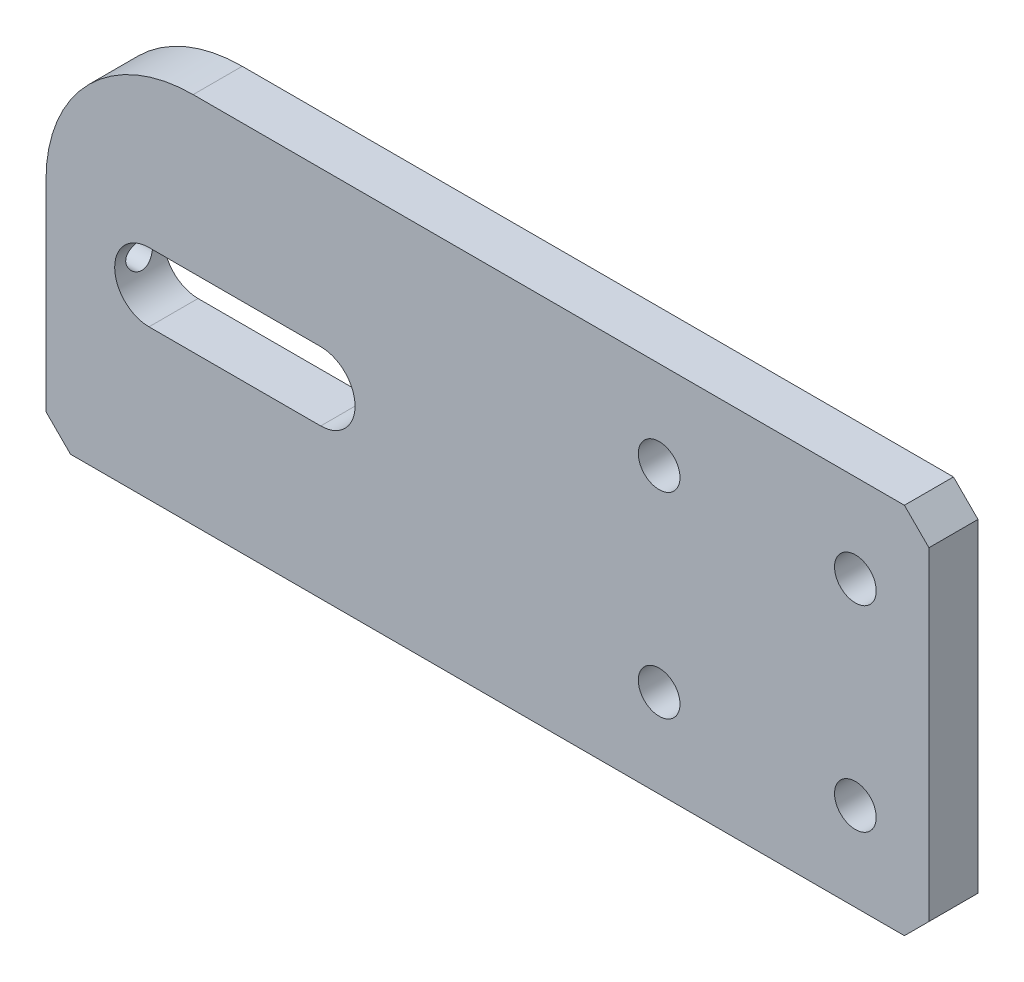
from build123d import *

# Parameters (mm, degrees)
EXTRUDE_1_DEPTH              = 5
HOLE_WIZARD_8_5_8_5_1_D      = 8.5
PATTERN_LINEAR_1_COUNT       = 2
PATTERN_LINEAR_1_PITCH       = 40
MIRROR_1_COPY_1_D            = 8.5
CUT_EXTRUDE_1_DEPTH          = 10
HOLE_WIZARD_5_5_5_5_1_REACH  = 186.035
HOLE_WIZARD_5_5_5_5_1_BORE_R = 2.75
CHAMFER_1_SIZE               = 5


with BuildPart() as part:
    # 草图2 → 凸台-拉伸1 (new, symmetric)
    with BuildSketch(Plane.XY):
        with BuildLine():
            Line((-60, 38), (90, 38))
            Line((90, 38), (90, -38))
            Line((90, -38), (-90, -38))
            Line((-90, -38), (-90, 8))
            ThreePointArc((-90, 8), (-81.213203436, 29.213203436), (-60, 38))
        make_face()
    extrude(amount=EXTRUDE_1_DEPTH, both=True)

    # Ø8.5 (8.5) 直径孔1 (through all)
    with Locations(Plane.XY.offset(5)):
        with Locations((75, 20)):
            hole_wizard_8_5_8_5_1 = Hole(HOLE_WIZARD_8_5_8_5_1_D / 2)

    # 阵列(线性)1: Ø8.5 (8.5) 直径孔1 ×2
    with Locations(*[(-i * PATTERN_LINEAR_1_PITCH, 0, 0) for i in range(1, PATTERN_LINEAR_1_COUNT)]):
        add(hole_wizard_8_5_8_5_1, mode=Mode.SUBTRACT)

    # 镜向1: Ø8.5 (8.5) 直径孔1 across plane
    add(hole_wizard_8_5_8_5_1.mirror(Plane.ZX), mode=Mode.SUBTRACT)

    # 镜向1 copy 1 (through all)
    with Locations(Plane(origin=(-40, 0, 5), x_dir=(1, 0, 0), z_dir=(0, 0, 1))):
        with Locations((75, -20)):
            Hole(MIRROR_1_COPY_1_D / 2)

    # 草图5 → 切除-拉伸1 (cut)
    with BuildSketch(Plane.XY.offset(5)):
        with BuildLine():
            Line((-69, 6.5), (-34, 6.5))
            ThreePointArc((-34, 6.5), (-27, -0.5), (-34, -7.5))
            Line((-34, -7.5), (-69, -7.5))
            ThreePointArc((-69, -7.5), (-76, -0.5), (-69, 6.5))
        make_face()
    extrude(amount=-CUT_EXTRUDE_1_DEPTH, mode=Mode.SUBTRACT)

    # Ø5.5 (5.5) 直径孔1 bore → Ø5.5 (5.5) 直径孔1 (cut, up to next)
    with BuildSketch(Plane.ZY.offset(90), mode=Mode.PRIVATE) as hole_wizard_5_5_5_5_1_sk1:
        with Locations((0, -0.5)):
            Circle(HOLE_WIZARD_5_5_5_5_1_BORE_R)
    hole_wizard_5_5_5_5_1_tool1 = extrude(hole_wizard_5_5_5_5_1_sk1.sketch, amount=-HOLE_WIZARD_5_5_5_5_1_REACH, mode=Mode.PRIVATE) & part.part
    add(hole_wizard_5_5_5_5_1_tool1.solids().sort_by_distance((-90, -0.5, 0))[0], mode=Mode.SUBTRACT)

    # 倒角1
    chamfer_1_edges = [part.edges().sort_by_distance(p)[0] for p in [
        (90, -38, 0),
        (-90, -38, 0),
        (90, 38, 0),
    ]]
    chamfer(chamfer_1_edges, length=CHAMFER_1_SIZE)


solid = part.part
